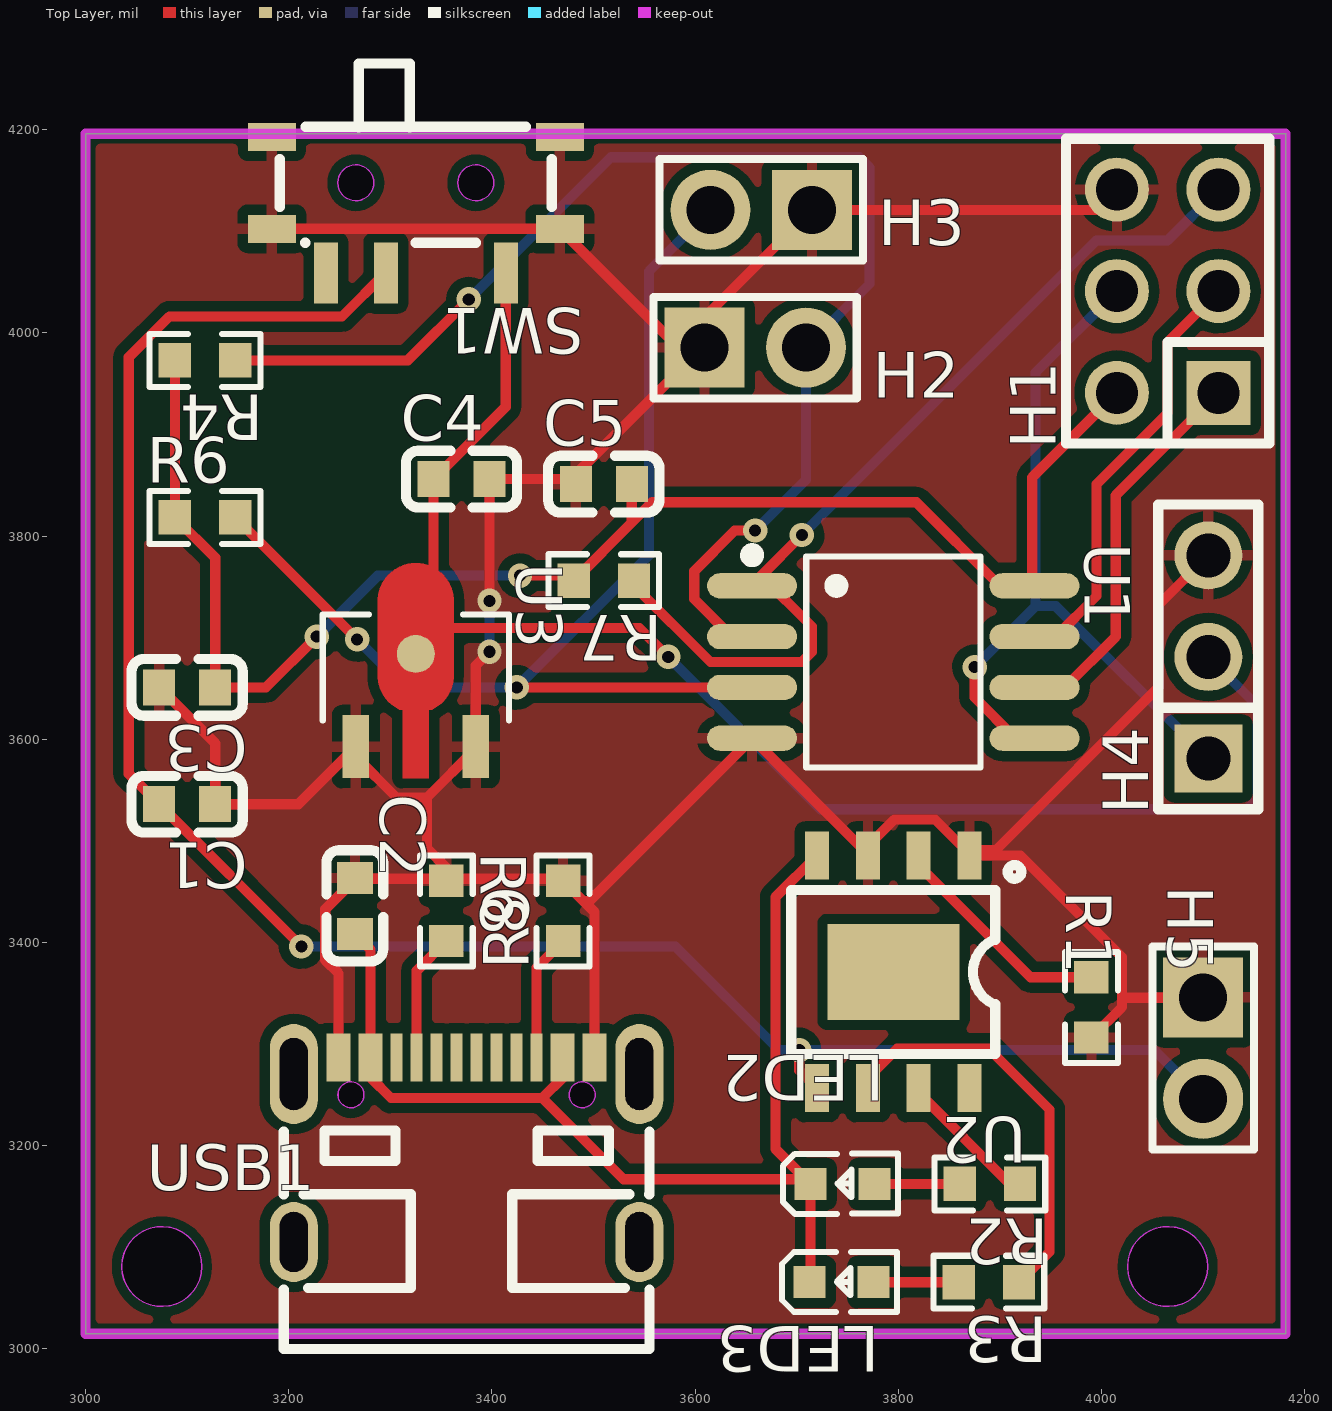
[diagram p0: Top Layer view]
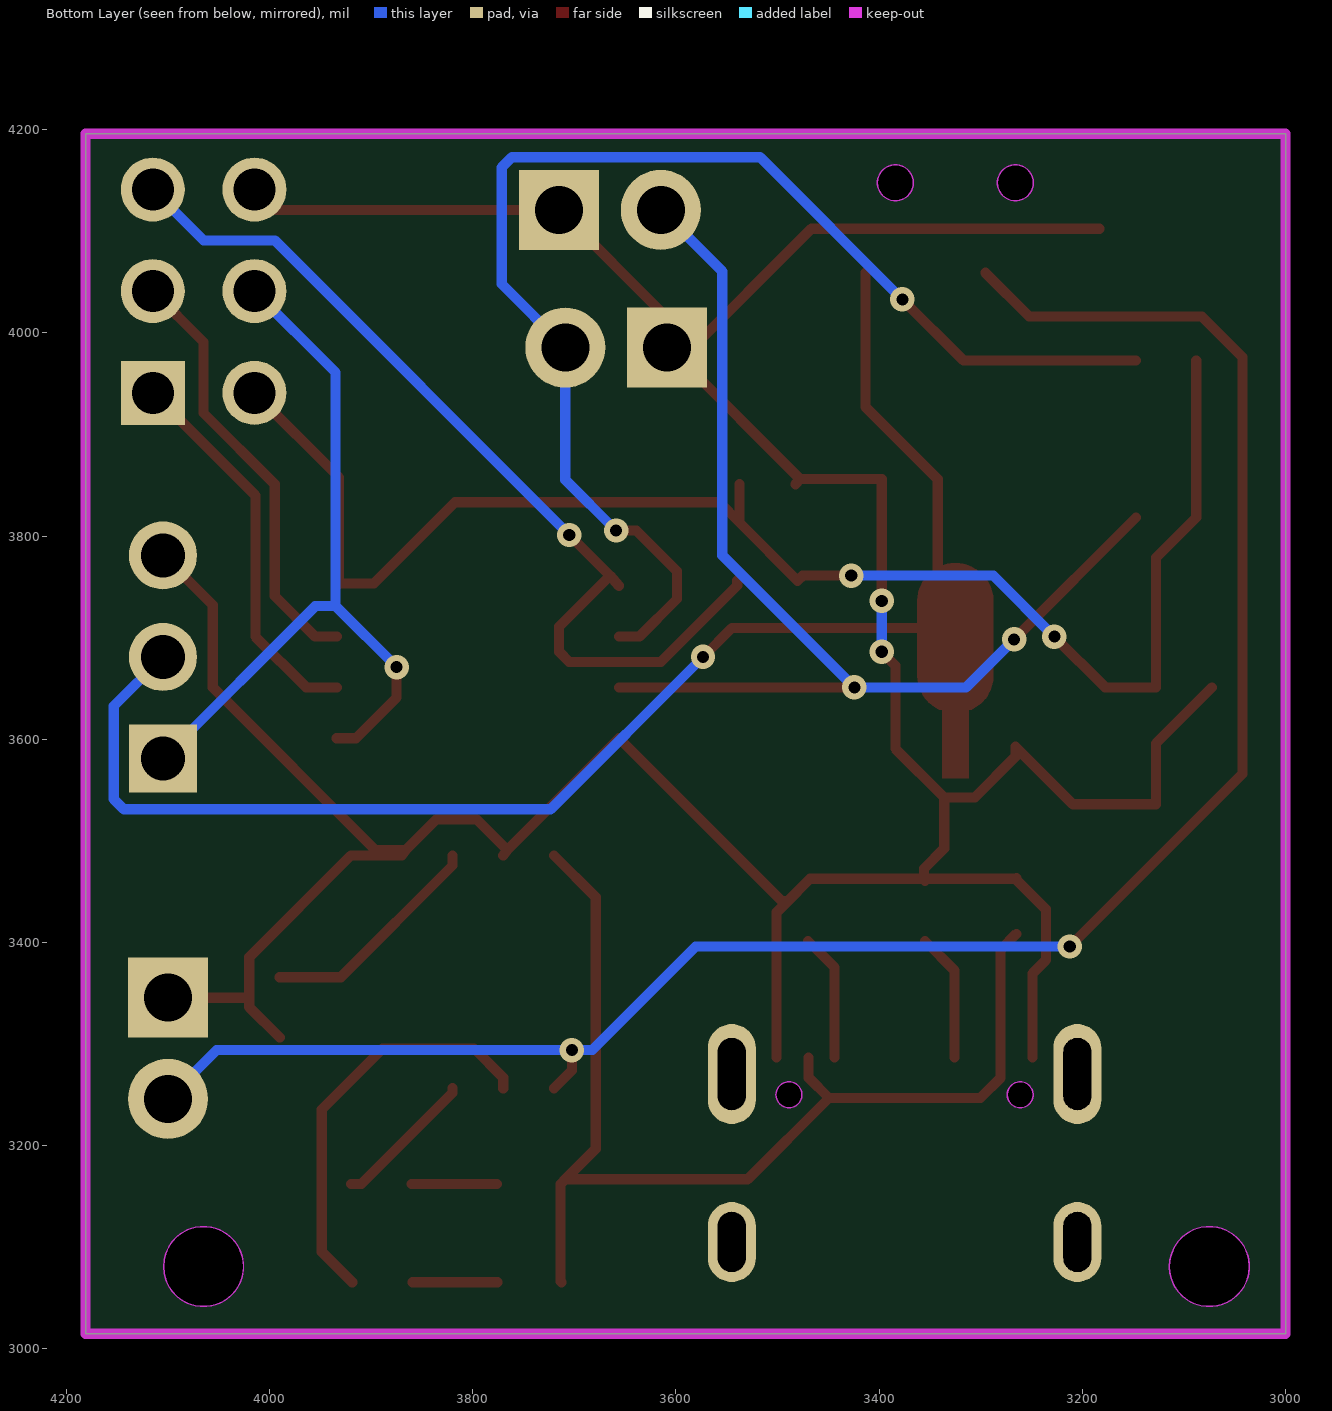
[diagram p1: Bottom Layer view, seen from below]
# Altium PCB MISC89049.pcbdoc
Units mil, origin at the board's own origin, x right, y up, seen from the top; angles counter-clockwise.
Board outline 1181.1 x 1181.1 mil, 2 copper layers (Top Layer, Bottom Layer), stack 62.206 mil thick; 25 components, 18 nets, 88 pads, 13 vias.

## Layer stack, top to bottom
Top Solder Mask Layer: solder mask 0.394, Dk 3.3
Top Layer: signal copper 1.379
Dielectric1: surface 59.449, FR4, Dk 4.5
Bottom Layer: signal copper 1.378
Bottom Solder Mask Layer: solder mask 0.394, Dk 3.3

## Board outline
3000,4196.02 3000,3014.92 4181.1,3014.92 4181.1,4196.02
cut-out: 3114.37,3081.02 cw(c3075,3081.02) 3035.63,3081.02 cw(c3075,3081.02)
cut-out: 4104.37,3081.02 cw(c4065,3081.02) 4025.63,3081.02 cw(c4065,3081.02)

## Design rules (kind name [scope] priority, off if disabled: settings)
BoardOutlineClearance copperThickness2oz_1 [All] p2 off: genericclearance=7.99 ignorepadtopadclearanceinfootprint=FALSE except(0: Arc-SplitContinuation Track-SplitContinuation SMDPad-SplitContinuation THPad-SplitContinuation Via-SplitContinuation Fill-SplitContinuation Region-SplitContinuation Poly-SplitContinuation Text-SplitContinuation Hole-SplitContinuation; 5.98: Arc-CutoutEdge Track-CutoutEdge SMDPad-CutoutEdge THPad-CutoutEdge Via-CutoutEdge Text-CutoutEdge; 6.9: Hole-OutlineEdge Hole-CutoutEdge; 10: Poly-OutlineEdge Poly-CutoutEdge; 11.81: Arc-OutlineEdge Track-OutlineEdge SMDPad-OutlineEdge THPad-OutlineEdge Via-OutlineEdge Fill-OutlineEdge Region-OutlineEdge Text-OutlineEdge Fill-CutoutEdge Region-CutoutEdge)
BoardOutlineClearance Plane_innerPlane_1 [All] p4 off: genericclearance=4.02 ignorepadtopadclearanceinfootprint=FALSE except(0: Arc-SplitContinuation Track-SplitContinuation SMDPad-SplitContinuation THPad-SplitContinuation Via-SplitContinuation Fill-SplitContinuation Region-SplitContinuation Poly-SplitContinuation Text-SplitContinuation Hole-SplitContinuation; 5.98: Arc-CutoutEdge Track-CutoutEdge SMDPad-CutoutEdge THPad-CutoutEdge Via-CutoutEdge Text-CutoutEdge; 6.9: Hole-OutlineEdge Hole-CutoutEdge; 10: Poly-OutlineEdge Poly-CutoutEdge; 11.81: Arc-OutlineEdge Track-OutlineEdge SMDPad-OutlineEdge THPad-OutlineEdge Via-OutlineEdge Fill-OutlineEdge Region-OutlineEdge Text-OutlineEdge Fill-CutoutEdge Region-CutoutEdge)
BoardOutlineClearance Copper_copperRegion_1 [All] p6 off: genericclearance=4.02 ignorepadtopadclearanceinfootprint=FALSE except(0: Arc-SplitContinuation Track-SplitContinuation SMDPad-SplitContinuation THPad-SplitContinuation Via-SplitContinuation Fill-SplitContinuation Region-SplitContinuation Poly-SplitContinuation Text-SplitContinuation Hole-SplitContinuation; 5.98: Arc-CutoutEdge Track-CutoutEdge SMDPad-CutoutEdge THPad-CutoutEdge Via-CutoutEdge Text-CutoutEdge; 6.9: Hole-OutlineEdge Hole-CutoutEdge; 10: Poly-OutlineEdge Poly-CutoutEdge; 11.81: Arc-OutlineEdge Track-OutlineEdge SMDPad-OutlineEdge THPad-OutlineEdge Via-OutlineEdge Fill-OutlineEdge Region-OutlineEdge Text-OutlineEdge Fill-CutoutEdge Region-CutoutEdge)
BoardOutlineClearance copperThickness1oz_1 [All] p8: genericclearance=4.02 ignorepadtopadclearanceinfootprint=FALSE except(0: Arc-SplitContinuation Track-SplitContinuation SMDPad-SplitContinuation THPad-SplitContinuation Via-SplitContinuation Fill-SplitContinuation Region-SplitContinuation Poly-SplitContinuation Text-SplitContinuation Hole-SplitContinuation; 5.98: Arc-CutoutEdge Track-CutoutEdge SMDPad-CutoutEdge THPad-CutoutEdge Via-CutoutEdge Text-CutoutEdge; 6.9: Hole-OutlineEdge Hole-CutoutEdge; 10: Poly-OutlineEdge Poly-CutoutEdge; 11.81: Arc-OutlineEdge Track-OutlineEdge SMDPad-OutlineEdge THPad-OutlineEdge Via-OutlineEdge Fill-OutlineEdge Region-OutlineEdge Text-OutlineEdge Fill-CutoutEdge Region-CutoutEdge)
Clearance copperThickness2oz [All] p1 off: gap=7.99 ignorepadtopadclearanceinfootprint=FALSE except(5.98: SMDPad-Track SMDPad-SMDPad THPad-Track SMDPad-THPad THPad-THPad Track-Via SMDPad-Via THPad-Via Via-Via Fill-SMDPad Region-SMDPad Fill-THPad Region-THPad Fill-Via Region-Via Fill-Fill Fill-Region Region-Region Arc-Track Arc-SMDPad Arc-THPad Arc-Via Fill-Arc Region-Arc Arc-Arc Text-Track SMDPad-Text Text-THPad Text-Via Fill-Text Region-Text Arc-Text Text-Text; 6.9: Hole-Track Hole-SMDPad Hole-THPad Hole-Via Fill-Hole Region-Hole Hole-Arc Hole-Text; 10: Poly-Track Poly-SMDPad Poly-THPad Poly-Via Poly-Fill Poly-Region Poly-Poly Poly-Arc Poly-Text Poly-Hole; 11.81: Fill-Track Region-Track)
Clearance Plane_innerPlane [All] p3 off: gap=4.02 ignorepadtopadclearanceinfootprint=FALSE except(5.98: SMDPad-Track SMDPad-SMDPad THPad-Track SMDPad-THPad THPad-THPad Track-Via SMDPad-Via THPad-Via Via-Via Fill-SMDPad Region-SMDPad Fill-THPad Region-THPad Fill-Via Region-Via Fill-Fill Fill-Region Region-Region Arc-Track Arc-SMDPad Arc-THPad Arc-Via Fill-Arc Region-Arc Arc-Arc Text-Track SMDPad-Text Text-THPad Text-Via Fill-Text Region-Text Arc-Text Text-Text; 6.9: Hole-Track Hole-SMDPad Hole-THPad Hole-Via Fill-Hole Region-Hole Hole-Arc Hole-Text; 10: Poly-Track Poly-SMDPad Poly-THPad Poly-Via Poly-Fill Poly-Region Poly-Poly Poly-Arc Poly-Text Poly-Hole; 11.81: Fill-Track Region-Track)
Clearance Copper_copperRegion [All] p5 off: gap=4.02 ignorepadtopadclearanceinfootprint=FALSE except(5.98: SMDPad-Track SMDPad-SMDPad THPad-Track SMDPad-THPad THPad-THPad Track-Via SMDPad-Via THPad-Via Via-Via Fill-SMDPad Region-SMDPad Fill-THPad Region-THPad Fill-Via Region-Via Fill-Fill Fill-Region Region-Region Arc-Track Arc-SMDPad Arc-THPad Arc-Via Fill-Arc Region-Arc Arc-Arc Text-Track SMDPad-Text Text-THPad Text-Via Fill-Text Region-Text Arc-Text Text-Text; 6.9: Hole-Track Hole-SMDPad Hole-THPad Hole-Via Fill-Hole Region-Hole Hole-Arc Hole-Text; 10: Poly-Track Poly-SMDPad Poly-THPad Poly-Via Poly-Fill Poly-Region Poly-Poly Poly-Arc Poly-Text Poly-Hole; 11.81: Fill-Track Region-Track)
Clearance copperThickness1oz [All] p7: gap=4.02 ignorepadtopadclearanceinfootprint=FALSE except(5.98: SMDPad-Track SMDPad-SMDPad THPad-Track SMDPad-THPad THPad-THPad Track-Via SMDPad-Via THPad-Via Via-Via Fill-SMDPad Region-SMDPad Fill-THPad Region-THPad Fill-Via Region-Via Fill-Fill Fill-Region Region-Region Arc-Track Arc-SMDPad Arc-THPad Arc-Via Fill-Arc Region-Arc Arc-Arc Text-Track SMDPad-Text Text-THPad Text-Via Fill-Text Region-Text Arc-Text Text-Text; 6.9: Hole-Track Hole-SMDPad Hole-THPad Hole-Via Fill-Hole Region-Hole Hole-Arc Hole-Text; 10: Poly-Track Poly-SMDPad Poly-THPad Poly-Via Poly-Fill Poly-Region Poly-Poly Poly-Arc Poly-Text Poly-Hole; 11.81: Fill-Track Region-Track)
DiffPairsRouting differentialPair [All] p1: maxlimit=6 minlimit=6 mostfreqgap=6 toplayer_minwidth=5 toplayer_prefwidth=10 toplayer_maxwidth=100 toplayer_mingap=6 toplayer_prefgap=6 toplayer_maxgap=6 bottomlayer_minwidth=5 bottomlayer_prefwidth=10 bottomlayer_maxwidth=100 bottomlayer_mingap=6 bottomlayer_prefgap=6 bottomlayer_maxgap=6 maxuncoupledlength=10
HoleToHoleClearance otherClearance [All] p1: gap=11.81 allowstackedmicrovias=TRUE
Length netLength [All] p1: minlimit=0 maxlimit=0
PasteMaskExpansion pasteMaskExpansion [All] p1: expansion=0
PlaneConnect innerPlane [All] p1: planeconnectstyle=Relief reliefexpansion=20 reliefentries=4 reliefconductorwidth=10 reliefairgap=10
PolygonConnect copperRegion [All] p1: connectstyle=Relief reliefconductorwidth=10 reliefentries=4 polygonreliefangle="90 Angle" airgapwidth=10 via.connectstyle=Relief via.reliefconductorwidth=10 via.reliefentries=4 via.polygonreliefangle="90 Angle" via.airgapwidth=10
RoutingVias viaSize [All] p1: holewidth=12.01 width=24.02 viastyle="Through Hole" minholewidth=11.81 minwidth=19.68 maxholewidth=248.03 maxwidth=393.7
SolderMaskExpansion solderMaskExpansion [IsVia] p1: expansion=-1000 istentingtop=TRUE
SolderMaskExpansion solderMaskExpansion [All] p2: expansion=2 istentingtop=FALSE
Width copperThickness2oz_2 [All] p1 off: maxlimit=100 minlimit=8 preferedwidth=10
Width copperThickness1oz_2 [All] p2: maxlimit=100 minlimit=5 preferedwidth=10

## Components (designator, comment, footprint, x,y, rotation, side; value= is the part's Value field where it differs from the comment)
C1 "1uF" C0603 3100,3536.02 r180 top
C2 "1uF" C0603 3265,3436.02 r270 top
C3 "1uF" C0603 3100,3651.02 r180 top
C4 "1uF" C0603 3370,3856.02 r0 top
C5 "100nF" C0603 3510,3851.02 r0 top
H1 "2.54-2*3" HDR-TH_6P-P2.54-V-R2-C3-S2.54_A2541WV-2X3P 4065,4041.02 r90 top
H2 "PZ254V-11-02P" HDR-TH_2P-P2.54-V-M 3659,3985.45 r0 top
H3 "PZ254V-11-02P" HDR-TH_2P-P2.54-V-M 3665,4121.02 r180 top
H4 "PZ254V-11-03P" HDR-TH_3P-P2.54-V-M 4105,3681.02 r90 top
H5 "PZ254V-11-02P" HDR-TH_2P-P2.54-V-M 4100,3296.02 r270 top
LED2 "LTST-C190KSKT" LED0603-RD 3745,3162.29 r0 top
LED3 "LTST-C190KSKT" LED0603-RD 3744.07,3065.6 r0 top
R1 "10kΩ" R0603 3990,3336.02 r90 top
R2 "1kΩ" R0603 3890,3162.29 r180 top
R3 "1kΩ" R0603 3889.07,3065.6 r180 top
R4 "10kΩ" R0603 3117.53,3972.88 r180 top
R6 "10kΩ" R0603 3117.53,3818.28 r0 top
R7 "10kΩ" R0603 3510,3756.02 r180 top
R8 "5.1kΩ" R0603 3355,3431.02 r270 top
R9 "5.1kΩ" R0603 3470,3431.02 r90 top
SW1 "MSK12C02" SW-TH_MSK12C02 3325,4126.02 r180 top
U1 "ATTINY85-20SU" SOIC-8_L5.3-W5.3-P1.27-LS8.0-BL 3795,3676.02 r270 top
U2 "TC4056A." ESOP-8_L4.9-W3.9-P1.27-LS6.0-BL-EP 3795,3371.02 r180 top
U3 "HT7333-A" SOT-89-3_L4.5-W2.5-P1.50-LS4.2-BR 3325,3646.02 r270 top
USB1 "MC-107D" USB-C-SMD_MC-107D 3375,3196.02 r0 top

## Footprints (in the part's own frame and the unit in brackets; to place one, negate y for a bottom-side part, rotate by r counter-clockwise, add the part's x,y. Pads: shape width x height; smd on the part's side, far side on the other; paste and mask are expansions set on the pad)
C0603 [mm]
  rect 0.8x0.9 smd: 1(-0.7,0) 2(0.7,0)
  silkscreen extent -1.39,-0.71 1.39,0.71
ESOP-8_L4.9-W3.9-P1.27-LS6.0-BL-EP [mm]
  rect 0.6x1.2 smd: 1(-1.905,-2.908) 2(-0.635,-2.908) 3(0.635,-2.908) 4(1.905,-2.908) 5(1.905,2.908) 6(0.635,2.908) 7(-0.635,2.908) 8(-1.905,2.908)
  rect 3.3x2.4 smd: 9(0,0)
  silkscreen extent -3.2,-2.67 2.55,2.05
HDR-TH_2P-P2.54-V-M [mm]
  rect 2x2 hole 1.2: 1(-1.27,0)
  round 2 hole 1.2: 2(1.27,0)
  silkscreen extent -2.54,-1.27 2.54,1.27
HDR-TH_3P-P2.54-V-M [mm]
  rect 1.7x1.7 hole 1.1: 1(-2.54,0)
  round 1.7 hole 1.1: 2(0,0) 3(2.54,0)
  silkscreen extent -3.81,-1.25 3.81,1.25
HDR-TH_6P-P2.54-V-R2-C3-S2.54_A2541WV-2X3P [mm]
  rect 1.6x1.6 hole 1.05: 1(-2.54,-1.27)
  round 1.6 hole 1.05: 2(-2.54,1.27) 3(0,-1.27) 4(0,1.27) 5(2.54,-1.27) 6(2.54,1.27)
  silkscreen extent -3.81,-2.54 3.81,2.54
LED0603-RD [mm]
  rect 0.8x0.8 smd: 1(-0.799,0) 2(0.799,0)
  silkscreen extent -1.49,-0.75 1.39,0.76
R0603 [mil]
  rect 31.75x34.02 smd paste-3937.01 mask+2: 1(-29.66,0) 2(29.66,0)
  silkscreen extent -55,-26 55,26
SOIC-8_L5.3-W5.3-P1.27-LS8.0-BL [mm]
  oval 0.63x2.25 smd: 1(-1.905,-3.53) 2(-0.635,-3.53) 3(0.635,-3.53) 4(1.905,-3.53) 5(1.905,3.53) 6(0.635,3.53) 7(-0.635,3.53) 8(-1.905,3.53)
  silkscreen extent -2.82,-3.68 2.64,2.18
SOT-89-3_L4.5-W2.5-P1.50-LS4.2-BR [mm]
  rect 1.575x0.672 smd: 1(1.356,-1.5) 3(1.356,1.5)
  round 0.95 smd: 2(-0.966,0)
  Top Layer region: -2.283,0.95 -0.429,0.95 -0.384,0.949 -0.34,0.946 -0.296,0.94 -0.252,0.933 -0.208,0.924 -0.165,0.912 -0.123,0.899 -0.081,0.884 -0.04,0.866 0,0.847 0.04,0.826 0.078,0.803 0.115,0.779 0.151,0.752 0.185,0.724 0.219,0.695 0.251,0.664 0.281,0.631 0.31,0.597 0.337,0.562 0.362,0.525 0.386,0.488 0.408,0.449 0.428,0.409 0.447,0.33 2.144,0.33 2.144,-0.33 0.447,-0.33 0.428,-0.409 0.408,-0.449 0.386,-0.488 0.362,-0.526 0.337,-0.562 0.31,-0.597 0.281,-0.631 0.251,-0.664 0.219,-0.695 0.185,-0.725 0.151,-0.753 0.115,-0.779 0.078,-0.804 0.04,-0.827 0,-0.848 -0.04,-0.867 -0.081,-0.884 -0.123,-0.899 -0.165,-0.913 -0.208,-0.924 -0.252,-0.934 -0.296,-0.941 -0.34,-0.946 -0.384,-0.949 -0.429,-0.95 -2.283,-0.95 -2.328,-0.949 -2.372,-0.946 -2.416,-0.941 -2.46,-0.934 -2.504,-0.924 -2.547,-0.913 -2.589,-0.899 -2.631,-0.884 -2.672,-0.867 -2.713,-0.848 -2.752,-0.827 -2.79,-0.804 -2.827,-0.779 -2.863,-0.753 -2.898,-0.725 -2.931,-0.695 -2.963,-0.664 -2.993,-0.631 -3.022,-0.597 -3.049,-0.562 -3.075,-0.526 -3.098,-0.488 -3.12,-0.449 -3.141,-0.409 -3.159,-0.369 -3.175,-0.327 -3.189,-0.285 -3.202,-0.242 -3.212,-0.199 -3.22,-0.155 -3.227,-0.111 -3.231,-0.067 -3.233,-0.022 -3.233,0.022 -3.231,0.067 -3.227,0.111 -3.22,0.155 -3.212,0.199 -3.202,0.242 -3.189,0.285 -3.175,0.327 -3.159,0.369 -3.141,0.409 -3.12,0.449 -3.098,0.488 -3.075,0.525 -3.049,0.562 -3.022,0.597 -2.993,0.631 -2.963,0.664 -2.931,0.695 -2.898,0.724 -2.863,0.752 -2.827,0.779 -2.79,0.803 -2.752,0.826 -2.713,0.847 -2.672,0.866 -2.631,0.884 -2.589,0.899 -2.547,0.912 -2.504,0.924 -2.46,0.933 -2.416,0.94 -2.372,0.946 -2.328,0.949
  silkscreen extent -1.95,-2.33 0.7,2.33
SW-TH_MSK12C02 [mm]
  rect 0.6x1.524 smd: 1(-2.25,1.7) 2(0.75,1.7) 3(2.25,1.7)
  rect 1.2x0.7 smd: 4(-3.6,-1.7) 4(-3.6,0.6) 4(3.6,-1.7) 4(3.6,0.6)
  Board Outline Layer circle w0.003: c-1.5,-0.55 r0.45
  Board Outline Layer circle w0.003: c1.5,-0.55 r0.45
  Board Outline Layer region: -1.95,-0.55 -1.905,-0.355 -1.78,-0.198 -1.6,-0.111 -1.4,-0.111 -1.219,-0.198 -1.094,-0.355 -1.05,-0.55 -1.05,-0.55 -1.094,-0.745 -1.219,-0.902 -1.4,-0.989 -1.6,-0.989 -1.78,-0.902 -1.905,-0.745 -1.95,-0.55
  Board Outline Layer region: -1.95,-0.55 -1.94,-0.457 -1.911,-0.367 -1.864,-0.286 -1.801,-0.216 -1.725,-0.16 -1.639,-0.122 -1.547,-0.103 -1.453,-0.103 -1.361,-0.122 -1.275,-0.16 -1.199,-0.216 -1.136,-0.286 -1.089,-0.367 -1.06,-0.457 -1.05,-0.55 -1.06,-0.644 -1.089,-0.733 -1.136,-0.815 -1.199,-0.885 -1.275,-0.94 -1.361,-0.978 -1.453,-0.998 -1.547,-0.998 -1.639,-0.978 -1.725,-0.94 -1.801,-0.885 -1.864,-0.815 -1.911,-0.733 -1.94,-0.644
  Board Outline Layer region: 1.05,-0.55 1.095,-0.355 1.22,-0.198 1.4,-0.111 1.6,-0.111 1.781,-0.198 1.906,-0.355 1.95,-0.55 1.95,-0.55 1.906,-0.745 1.781,-0.902 1.6,-0.989 1.4,-0.989 1.22,-0.902 1.095,-0.745 1.05,-0.55
  Board Outline Layer region: 1.05,-0.55 1.06,-0.457 1.089,-0.367 1.136,-0.286 1.199,-0.216 1.275,-0.16 1.361,-0.122 1.453,-0.103 1.547,-0.103 1.639,-0.122 1.725,-0.16 1.801,-0.216 1.864,-0.286 1.911,-0.367 1.94,-0.457 1.95,-0.55 1.94,-0.644 1.911,-0.733 1.864,-0.815 1.801,-0.885 1.725,-0.94 1.639,-0.978 1.547,-0.998 1.453,-0.998 1.361,-0.978 1.275,-0.94 1.199,-0.885 1.136,-0.815 1.089,-0.733 1.06,-0.644
  Multi-Layer board cut-out: -1.95,-0.55 -1.905,-0.355 -1.78,-0.198 -1.6,-0.111 -1.4,-0.111 -1.219,-0.198 -1.094,-0.355 -1.05,-0.55 -1.05,-0.55 -1.094,-0.745 -1.219,-0.902 -1.4,-0.989 -1.6,-0.989 -1.78,-0.902 -1.905,-0.745 -1.95,-0.55
  Multi-Layer board cut-out: 1.05,-0.55 1.095,-0.355 1.22,-0.198 1.4,-0.111 1.6,-0.111 1.781,-0.198 1.906,-0.355 1.95,-0.55 1.95,-0.55 1.906,-0.745 1.781,-0.902 1.6,-0.989 1.4,-0.989 1.22,-0.902 1.095,-0.745 1.05,-0.55
  silkscreen extent -3.4,-3.53 3.4,0.95
USB-C-SMD_MC-107D [mm]
  oval 1.2x2 hole 0.7 slot 1.5 at 90 deg: 0(-4.32,-2.308) 0(4.32,-2.308)
  oval 1.2x2.5 hole 0.7 slot 1.8 at 90 deg: 0(-4.32,1.892) 0(4.32,1.892)
  rect 0.6x1.2 smd paste-100 mask+0.051: A1B12(-3.2,2.308) A4B9(-2.4,2.308) B1A12(3.2,2.308) B4A9(2.4,2.308)
  rect 0.3x1.2 smd paste-100 mask+0.051: A5(-1.25,2.308) A6(-0.25,2.308) A7(0.25,2.308) A8(1.25,2.308) B5(1.75,2.308) B6(0.75,2.308) B7(-0.75,2.308) B8(-1.75,2.308)
  Board Outline Layer circle w0.003: c2.89,1.372 r0.325
  Board Outline Layer circle w0.003: c-2.89,1.372 r0.325
  Board Outline Layer region: 3.215,1.372 3.183,1.231 3.093,1.118 2.962,1.055 2.818,1.055 2.687,1.118 2.597,1.231 2.565,1.372 2.565,1.372 2.597,1.513 2.687,1.626 2.818,1.689 2.962,1.689 3.093,1.626 3.183,1.513 3.215,1.372
  Board Outline Layer region: 3.215,1.372 3.206,1.294 3.178,1.221 3.133,1.156 3.075,1.105 3.005,1.068 2.929,1.049 2.851,1.049 2.775,1.068 2.705,1.105 2.647,1.156 2.602,1.221 2.574,1.294 2.565,1.372 2.574,1.45 2.602,1.523 2.647,1.587 2.705,1.639 2.775,1.676 2.851,1.695 2.929,1.695 3.005,1.676 3.075,1.639 3.133,1.587 3.178,1.523 3.206,1.45
  Board Outline Layer region: -2.565,1.372 -2.597,1.231 -2.687,1.118 -2.818,1.055 -2.962,1.055 -3.093,1.118 -3.183,1.231 -3.215,1.372 -3.215,1.372 -3.183,1.513 -3.093,1.626 -2.962,1.689 -2.818,1.689 -2.687,1.626 -2.597,1.513 -2.565,1.372
  Board Outline Layer region: -2.565,1.372 -2.574,1.294 -2.602,1.221 -2.647,1.156 -2.705,1.105 -2.775,1.068 -2.851,1.049 -2.929,1.049 -3.005,1.068 -3.075,1.105 -3.133,1.156 -3.178,1.221 -3.206,1.294 -3.215,1.372 -3.206,1.45 -3.178,1.523 -3.133,1.587 -3.075,1.639 -3.005,1.676 -2.929,1.695 -2.851,1.695 -2.775,1.676 -2.705,1.639 -2.647,1.587 -2.602,1.523 -2.574,1.45
  Multi-Layer board cut-out: 3.215,1.372 3.183,1.231 3.093,1.118 2.962,1.055 2.818,1.055 2.687,1.118 2.597,1.231 2.565,1.372 2.565,1.372 2.597,1.513 2.687,1.626 2.818,1.689 2.962,1.689 3.093,1.626 3.183,1.513 3.215,1.372
  Multi-Layer board cut-out: -2.565,1.372 -2.597,1.231 -2.687,1.118 -2.818,1.055 -2.962,1.055 -3.093,1.118 -3.183,1.231 -3.215,1.372 -3.215,1.372 -3.183,1.513 -3.093,1.626 -2.962,1.689 -2.818,1.689 -2.687,1.626 -2.597,1.513 -2.565,1.372
  silkscreen extent -4.57,-4.98 4.57,0.48

## Via types
v1: diameter 24.02, hole 12, Top Layer to Bottom Layer, 13 vias

## Nets (pads, with @x,y where several pads share a name; then routed paths per layer and width w, separated by ;. In a path a pad name is that pad's centre, name@x,y a point inside that pad or via, vN(x,y) a via of type N, cw(c..) or ccw(c..) an arc to the next point about the centre after c; other vN are vias at no path point)
$1N741: R1.2 U2.2 | length 225.4
  Top Layer w10: U2.2 3820,3475.68 3930,3365.68 R1.2
$1N844: R2.1 U2.7 | length 141.4
  Top Layer w10: U2.7 3820,3251.95 3909.66,3162.29 R2.1
$1N935: LED2.2 R2.2 | length 83.9
  Top Layer w10: LED2.2 R2.2
$1N1062: LED3.2 R3.2 | length 83.9
  Top Layer w10: LED3.2 R3.2
$1N1066: R3.1 U2.6 | length 408.3
  Top Layer w10: U2.6 3770,3266.87 3798.73,3295.6 3888.73,3295.6 3948.73,3235.6 3948.73,3095.6 R3.1
$1N2613: H3.2 R6.2 U1.3 | length 1127
  Top Layer w10: R6.2 v1(3267.19,3698.28) ; v1(3424.45,3651.02) U1.3
  Bottom Layer w10: v1(3267.19,3698.28) 3314.45,3651.02 v1(3424.45,3651.02) 3554.45,3781.02 3554.45,4060.47 H3.2
$1N2918: H2.2 R4.1 U1.2 | length 1291.7
  Top Layer w10: R4.1 3317.19,3972.88 v1(3377.19,4032.88) ; U1.2 3636.02,3701.02 3599,3738.04 3599,3765.45 3639,3805.45 v1(3659,3805.45)
  Bottom Layer w10: v1(3377.19,4032.88) 3517.19,4172.88 3761.56,4172.88 3771.56,4162.88 3771.56,4048.01 H2.2 3709,3855.45 v1(3659,3805.45)
$1N3030: R8.2 USB1.A5 | length 126.6
  Top Layer w10: USB1.A5 3325.79,3372.15 R8.2
$1N3210: R9.1 USB1.B5 | length 125.3
  Top Layer w10: USB1.B5 3443.9,3375.26 R9.1
$1N3592: H1.5 R7.1 U1.1 | length 931.9
  Top Layer w10: R7.1 3539.66,3751.36 3615,3676.02 3705,3676.02 3715,3686.02 3715,3711.02 U1.1@3665,3761.02 ; U1.1 U1.1@3665,3761.02 ; v1(3705,3801.02) U1.1@3665,3761.02
  Bottom Layer w10: v1(3705,3801.02) 3995,4091.02 4065,4091.02 H1.5
$1N3598: H1.4 H4.1 U1.5 | length 765.7
  Top Layer w10: v1(3875,3671.02) 3875,3641.02 3915,3601.02 U1.5
  Bottom Layer w10: v1(3875,3671.02) 3935,3731.02 ; H1.4 3935,3961.02 3935,3731.02 ; H4.1 3955,3731.02 3935,3731.02
$1N3838: H1.1 U1.6 | length 382.6
  Top Layer w10: U1.6 3963.98,3651.02 4013.98,3701.02 4013.98,3840 H1.1
$1N3863: H1.3 U1.7 | length 427.3
  Top Layer w10: U1.7 3955,3701.02 3995,3741.02 3995,3851.02 4065,3921.02 4065,3991.02 H1.3
+3.3V: C3.1 C5.2 H1.2 R4.2 R6.1 R7.2 U1.8 | length 1518.4
  Top Layer w10: R4.2 R6.1 3127.56,3778.59 C3.1 3177.56,3651.02 v1(3227.56,3701.02) ; v1(3427.56,3761.02) 3475.34,3761.02 R7.2 3537.56,3813.24 ; C5.2 3537.56,3813.24 ; U1.8 U1.8@3931.76,3753.24 ; H1.2 3931.76,3857.78 U1.8@3931.76,3753.24 ; 3537.56,3813.24 3557.56,3833.24 3817.56,3833.24 3897.56,3753.24 U1.8@3931.76,3753.24
  Bottom Layer w10: v1(3227.56,3701.02) 3287.56,3761.02 v1(3427.56,3761.02)
+5V: C2.2 LED2.1 LED3.1 U2.4 USB1.A4B9 USB1.B4A9 | length 1117.8
  Top Layer w10: C2.2 3280.51,3392.95 USB1.A4B9 3280.51,3266.89 3300.51,3246.89 3449.49,3246.89 ; USB1.B4A9 3469.49,3266.89 3449.49,3246.89 ; LED3.1 3713.53,3066.53 LED2.1 LED2.1@3708.92,3166.89 ; U2.4 3678.92,3444.44 3678.92,3196.89 LED2.1@3708.92,3166.89 ; 3449.49,3246.89 3529.49,3166.89 LED2.1@3708.92,3166.89
+5VBAT: C4.1 H4.2 SW1.1 U3.2 | length 1452.8
  Top Layer w10: U3.2@3324.99,3699.42 3334.99,3709.42 ; SW1.1 3413.58,3927.16 C4.1 3342.44,3716.86 3334.99,3709.42 ; v1(3573.39,3681.02) 3544.99,3709.42 3334.99,3709.42
  Bottom Layer w10: v1(3573.39,3681.02) 3723.39,3531.02 4143.39,3531.02 4153.39,3541.02 4153.39,3632.63 H4.2
+5VBATOUT: C1.2 H5.2 SW1.2 U2.5 | length 1932.4
  Top Layer w10: v1(3212.44,3396.02) C1.2 3042.44,3566.02 3042.44,3976.02 3082.48,4016.06 3252.44,4016.06 SW1.2 ; v1(3702.44,3294.08) 3702.44,3274.08 U2.5
  Bottom Layer w10: v1(3212.44,3396.02) 3580.5,3396.02 3682.44,3294.08 v1(3702.44,3294.08) 4051.94,3294.08 H5.2
GND: C1.1 C2.1 C3.2 C4.2 C5.1 H1.6 H2.1 H3.1 H4.3 H5.1 R1.1 R8.1 R9.2 SW1.4 U1.4 U2.1 U2.3 U3.1 U3.3 USB1.A1B12 USB1.B1A12 | length 3934.1
  Top Layer w10: C3.2 3127.56,3595.9 C1.1 3209.34,3536.02 U3.1 3265.95,3582.63 3305.95,3542.63 3335.95,3542.63 ; SW1.4@3183.27,4102.4 3466.73,4102.4 3593.11,3976.02 H2.1@3597.56,3976.02 ; USB1.A1B12 3249.01,3369.56 3235.95,3382.63 3235.95,3432.63 C2.1@3265.95,3462.63 ; C2.1 C2.1@3265.95,3462.63 ; R8.1 R8.1@3355.95,3462.63 ; v1(3397.56,3686.13) 3384.05,3672.63 U3.3 3384.05,3590.74 3335.95,3542.63 ; v1(3397.56,3736.13) C4.2 C5.1@3477.56,3856.02 ; C5.1 C5.1@3477.56,3856.02 ; USB1.B1A12 3500.98,3429.7 3490,3440.68 ; U2.3 U2.3@3766.02,3491.02 ; R1.1 4020,3336.36 4020,3345.52 ; H1.6 3995,4121.02 H3.1 3609,4015.02 H2.1 H2.1@3597.56,3976.02 ; H5.1 4099.5,3345.52 4020,3345.52 ; H4.3 4056.02,3732.04 4056.02,3651.02 3896.02,3491.02 U2.1@3866.02,3491.02 ; C2.1@3265.95,3462.63 R8.1@3355.95,3462.63 ; 3335.95,3542.63 3335.95,3492.63 3355.95,3472.63 R8.1@3355.95,3462.63 ; R8.1@3355.95,3462.63 3468.05,3462.63 R9.2 3490,3440.68 ; C5.1@3477.56,3856.02 H2.1@3597.56,3976.02 ; 3490,3440.68 3495.68,3440.68 U1.4 U2.3@3766.02,3491.02 ; U2.3@3766.02,3491.02 3796.02,3521.02 3836.02,3521.02 U2.1@3866.02,3491.02 ; U2.1@3866.02,3491.02 U2.1 3920,3485.52 4020,3385.52 4020,3345.52
  Bottom Layer w10: v1(3397.56,3686.13) v1(3397.56,3736.13)
pads on no net: SW1.3 U2.8 U2.9 USB1.0 USB1.A6 USB1.A7 USB1.A8 USB1.B6 USB1.B7 USB1.B8

## Polygon pours and split planes (outlines as drawn)
GND on Top Layer (solid, remove dead copper, pour order 0): 3000,4196.02 3000,3014.92 4181.1,3014.92 4181.1,4196.02

## Keep-outs
Board Outline Layer:
  region: 3114.37,3081.02 cw(c3075,3081.02) 3035.63,3081.02 cw(c3075,3081.02)
  circle w0.1: c3075,3081.02 r39.37
  region: 3114.37,3081.02 3114,3075.66 3112.91,3070.4 3111.11,3065.34 3108.64,3060.56 3105.54,3056.18 3101.87,3052.25 3097.7,3048.86 3093.11,3046.06 3088.18,3043.92 3083.01,3042.47 3077.69,3041.74 3072.31,3041.74 3066.99,3042.47 3061.82,3043.92 3056.89,3046.06 3052.3,3048.86 3048.13,3052.25 3044.46,3056.18 3041.36,3060.56 3038.89,3065.34 3037.09,3070.4 3036,3075.66 3035.63,3081.02 3036,3086.38 3037.09,3091.64 3038.89,3096.71 3041.36,3101.48 3044.46,3105.87 3048.13,3109.79 3052.3,3113.19 3056.89,3115.98 3061.82,3118.12 3066.99,3119.57 3072.31,3120.3 3077.69,3120.3 3083.01,3119.57 3088.18,3118.12 3093.11,3115.98 3097.7,3113.19 3101.87,3109.79 3105.54,3105.87 3108.64,3101.48 3111.11,3096.71 3112.91,3091.64 3114,3086.38
  region: 4104.37,3081.02 cw(c4065,3081.02) 4025.63,3081.02 cw(c4065,3081.02)
  circle w0.1: c4065,3081.02 r39.37
  region: 4104.37,3081.02 4104,3075.66 4102.91,3070.4 4101.11,3065.34 4098.64,3060.56 4095.54,3056.18 4091.87,3052.25 4087.7,3048.86 4083.11,3046.06 4078.18,3043.92 4073.01,3042.47 4067.69,3041.74 4062.31,3041.74 4056.99,3042.47 4051.82,3043.92 4046.89,3046.06 4042.3,3048.86 4038.13,3052.25 4034.46,3056.18 4031.36,3060.56 4028.89,3065.34 4027.09,3070.4 4026,3075.66 4025.63,3081.02 4026,3086.38 4027.09,3091.64 4028.89,3096.71 4031.36,3101.48 4034.46,3105.87 4038.13,3109.79 4042.3,3113.19 4046.89,3115.98 4051.82,3118.12 4056.99,3119.57 4062.31,3120.3 4067.69,3120.3 4073.01,3119.57 4078.18,3118.12 4083.11,3115.98 4087.7,3113.19 4091.87,3109.79 4095.54,3105.87 4098.64,3101.48 4101.11,3096.71 4102.91,3091.64 4104,3086.38
  lines w10: 3000,3014.92 3000,4196.02 4181.1,4196.02 4181.1,3014.92 3000,3014.92

## Silkscreen, mask and mechanical layers (free items; w line width, h text height)
Mechanical Layer:
  circle w0.1: c3075,3081.02 r39.37
  circle w0.1: c4065,3081.02 r39.37